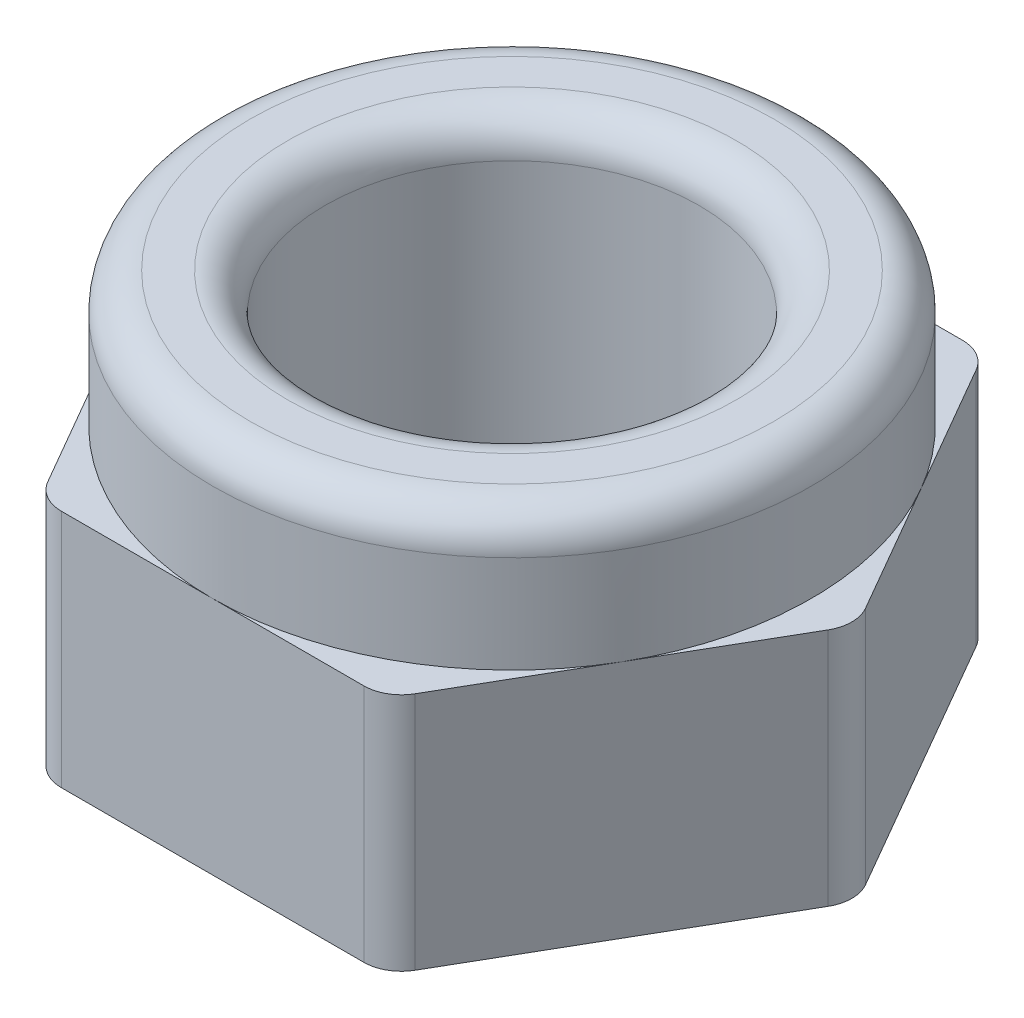
from build123d import *

# Parameters (mm, degrees)
SKETCH_1_R      = 2.5
EXTRUDE_1_DEPTH = 3.2
SKETCH_2_R      = 4
SKETCH_2_R_2    = 2.5
EXTRUDE_2_DEPTH = 1.8
FILLET_3_R      = 0.5


with BuildPart() as part:
    # 草图1 → 凸台-拉伸1 (new body)
    with BuildSketch(Plane(origin=(0, 0, 0), x_dir=(1, 0, 0), z_dir=(0, 1, 0))):
        Polygon((4.618802154, 0), (2.309401077, 4), (-2.309401077, 4), (-4.618802154, 0), (-2.309401077, -4), (2.309401077, -4), align=None)
        with Locations(Location((0, 0, 0), (0, 0, 270))):
            Circle(SKETCH_1_R, mode=Mode.SUBTRACT)
    extrude(amount=EXTRUDE_1_DEPTH)

    # 草图2 → 凸台-拉伸2 (add)
    with BuildSketch(Plane(origin=(0, 3.2, 0), x_dir=(1, 0, 0), z_dir=(0, 1, 0))):
        with Locations(Location((0, 0, 0), (0, 0, 270))):
            Circle(SKETCH_2_R)
        with Locations(Location((0, 0, 0), (0, 0, 270))):
            Circle(SKETCH_2_R_2, mode=Mode.SUBTRACT)
    extrude(amount=EXTRUDE_2_DEPTH)

    # 圆角3
    fillet_3_edges = [part.edges().sort_by_distance(p)[0] for p in [
        (2.309401077, 1.6, 4),
        (-2.309401077, 1.6, 4),
        (-4.618802154, 1.6, 0),
        (-2.309401077, 1.6, -4),
        (2.309401077, 1.6, -4),
        (4.618802154, 1.6, 0),
        (0, 5, -4),
        (0, 5, -2.5),
    ]]
    fillet(fillet_3_edges, radius=FILLET_3_R)


solid = part.part
